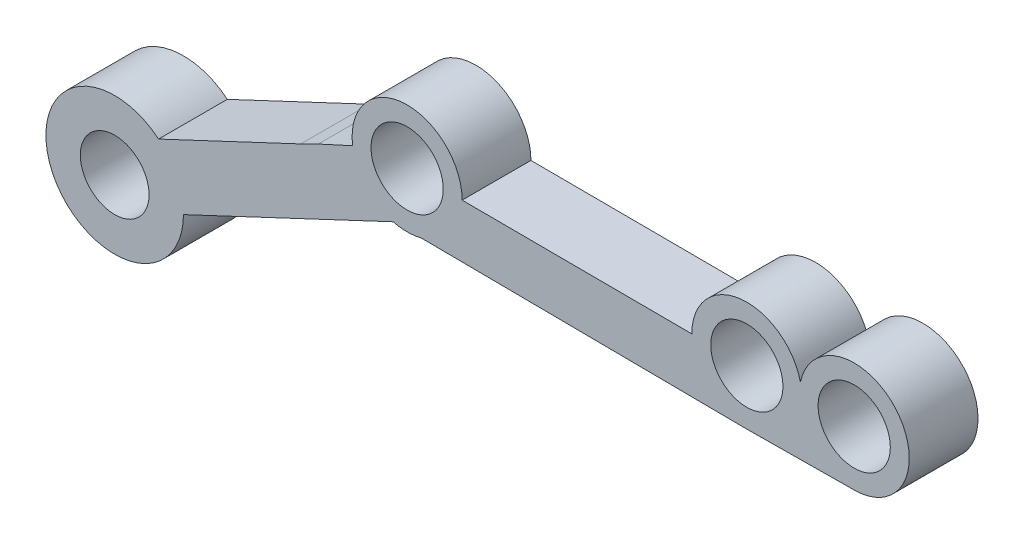
SolidWorks part; units mm, degrees
ref_plane "Front Plane" through (0, 0, 0) normal (0, 0, 1) x (1, 0, 0)
ref_plane "Top Plane" through (0, 0, 0) normal (0, 1, 0) x (1, 0, 0)
ref_plane "Right Plane" through (0, 0, 0) normal (1, 0, 0) x (0, 0, -1)
other "Configuration Table"
sketch "Sketch1" plane through (0, 0, 0) normal (0, 0, 1) x (1, 0, 0)
  line L0 (0, 0) -> (34, 0)
  line L1 (0, 0) -> (0, -15) construction
  line L2 (0, -15) -> (0, 0) construction
  line L3 (-12.0934, -8.0179) -> (-9.4868, -9.5228)
  line L4 (0, -5) -> (34, -5)
  line L5 (35, -4) -> (35, -1)
  arc A0 (0, 0) -> (-12.4215, -6.5913) centre (0, -15) ccw
  arc A1 (0, -5) -> (-8.1698, -9.2334) centre (0, -15) ccw
  arc A2 (34, 0) -> (35, -1) centre (34, -1) cw
  arc A3 (34, -5) -> (35, -4) centre (34, -4) ccw
  arc A4 (-12.4215, -6.5913) -> (-12.0934, -8.0179) centre (-11.5934, -7.1519) ccw
  arc A5 (-8.1698, -9.2334) -> (-9.4868, -9.5228) centre (-8.9868, -8.6567) cw
  dimension "D1" = 1
  dimension "D2" = 1
  dimension "D3" = 1
  dimension "D4" = 1
extrude "Boss-Extrude1" add sketch "Sketch1" along normal blind 5
sketch "Sketch2" plane through (0, 0, 5) normal (0, 0, 1) x (1, 0, 0)
  line L0 (28.5419, -2.571) -> (32.6338, -2.571) construction
  line L1 (-9.5871, -6.6866) -> (-10.7901, -8.7703) construction
  line L2 (-12.0934, -8.0179) -> (-9.4868, -9.5228) construction
  line L3 (32.6338, -2.571) -> (24.6949, -2.571) construction
  circle A0 centre (32.6338, -2.571) radius 1.5
  circle A3 centre (-9.5871, -6.6866) radius 1.5
  circle A4 centre (24.6949, -2.571) radius 1.5
sketch "Sketch3" plane through (0, 0, 0) normal (0, 0, -1) x (-1, 0, 0)
  line L0 (-35, -2.5) -> (0, -2.5) construction
  line L1 (-35, -4) -> (-35, -1) construction
  circle A0 centre (0, -2.5) radius 2.5
extrude "Cut-Extrude3" cut sketch "Sketch3" against normal blind 10
extrude "Cut-Extrude4" cut sketch "Sketch2" against normal blind 7
sketch "Sketch4" plane through (0, 0, 5) normal (0, 0, 1) x (1, 0, 0)
  line L0 (24.6949, -2.571) -> (16.6949, -2.571) construction
  circle A0 centre (16.6949, -2.571) radius 2.5
sketch "Sketch5" plane through (0, 0, 0) normal (0, 0, -1) x (-1, 0, 0)
  circle A0 centre (0, -2.5) radius 4
extrude "Boss-Extrude2" add sketch "Sketch5" against normal blind 5
sketch "Sketch6" plane through (0, 0, 5) normal (0, 0, 1) x (1, 0, 0)
  line L0 (35, -2.5) -> (13.021, -2.5) construction
  line L1 (35, -4) -> (35, -1) construction
  line L2 (16.6906, -2.5) -> (16.6906, -5) construction
  line L3 (3.1225, -5) -> (34, -5) construction
  circle A0 centre (16.6906, -2.5) radius 4
extrude "Boss-Extrude3" add sketch "Sketch6" against normal through all
sketch "Sketch7" plane through (0, 0, 5) normal (0, 0, 1) x (1, 0, 0)
  line L0 (35, -2.5) -> (32.5, -2.5)
  line L1 (35, -4) -> (35, -1) construction
  circle A0 centre (32.5, -2.5) radius 4
  line M5 (34, 0) -> (19.8131, 0)
  line M17 (19.8131, -5) -> (34, -5)
  arc M18 (34, -5) -> (35, -4) centre (34, -4) ccw
  line M19 (35, -4) -> (35, -1)
  arc M20 (35, -1) -> (34, 0) centre (34, -1) ccw
extrude "Boss-Extrude4" add sketch "Sketch7" against normal through all contours A0 M17 M5 M20 M19 M18
sketch "Sketch9" plane through (0, 0, 5) normal (0, 0, 1) x (1, 0, 0)
  circle A0 centre (-9.5871, -6.6866) radius 4
extrude "Boss-Extrude5" add sketch "Sketch9" against normal through all
sketch "Sketch10" plane through (0, 0, 5) normal (0, 0, 1) x (1, 0, 0)
  circle A0 centre (0, -2.5) radius 2.625
  circle A1 centre (-9.5871, -6.6866) radius 2.625
  circle A2 centre (16.6906, -2.5) radius 2.5
  circle A3 centre (32.5, -2.5) radius 2.625
extrude "Cut-Extrude5" cut sketch "Sketch10" against normal through all
sketch "Sketch11" plane through (0, 0, 5) normal (0, 0, 1) x (1, 0, 0)
  circle A0 centre (24.6949, -2.571) radius 4
  circle A1 centre (24.6949, -2.571) radius 2.5
extrude "Boss-Extrude6" add sketch "Sketch11" against normal through all contours A0
sketch "Sketch12" plane through (0, 0, 5) normal (0, 0, 1) x (1, 0, 0)
  circle A0 centre (24.6949, -2.571) radius 2.625
extrude "Cut-Extrude6" cut sketch "Sketch12" against normal through all
sketch "Sketch13" plane through (0, 0, 5) normal (0, 0, 1) x (1, 0, 0)
  circle A0 centre (16.6906, -2.5) radius 4
extrude "Boss-Extrude7" add sketch "Sketch13" against normal through all
sketch "Sketch14" plane through (0, 0, 5) normal (0, 0, 1) x (1, 0, 0)
  line L0 (13.5681, 0) -> (19.8131, 0)
  line L1 (19.8131, 0) -> (19.6082, 3.1014)
  line L2 (19.6082, 3.1014) -> (13.5681, 2.8442)
  line L3 (13.5681, 2.8442) -> (12.582, 1.2873)
  line L4 (12.582, 1.2873) -> (13.5681, 0)
  line L5 (13.5681, -5) -> (19.8131, -5)
  line L6 (3.1225, -5) -> (13.5681, -5) construction
  line L7 (19.8131, -5) -> (20.9346, -7.6449)
  line L8 (20.9346, -7.6449) -> (15.4424, -9.366)
  line L9 (15.4424, -9.366) -> (11.6327, -7.6449)
  line L10 (11.6327, -7.6449) -> (13.5681, -5)
  arc A0 (13.5681, -5) -> (19.8131, -5) centre (16.6906, -2.5) ccw construction
extrude "Cut-Extrude7" cut sketch "Sketch14" against normal through all
sketch "Sketch15" plane through (0, 0, 5) normal (0, 0, 1) x (1, 0, 0)
  line L0 (-8.7058, -2.7849) -> (-7.6075, 0.7948)
  line L1 (-7.6075, 0.7948) -> (-3.3982, -0.39)
  line L2 (24.6949, -2.571) -> (16.6949, -2.571) construction
  line L3 (4, -2.5) -> (20.6949, -2.571)
  line L4 (21.6305, 0) -> (5.4994, 2.1913)
  line L5 (5.4994, 2.1913) -> (3.1225, 0)
  line L6 (27.7592, 0) -> (28.4537, 2.5282)
  line L7 (28.4537, 2.5282) -> (29.3775, 0)
  arc A0 (-3.3982, -0.39) -> (-2.7655, -5.39) centre (0, -2.5) ccw
  arc A1 (-2.7655, -5.39) -> (-5.5871, -6.7064) centre (0, -15) ccw construction
  arc A2 (-8.7058, -2.7849) -> (-5.5871, -6.7064) centre (-9.5871, -6.6866) cw
  arc A3 (-8.7058, -2.7849) -> (-5.5871, -6.7064) centre (-9.5871, -6.6866) ccw construction
  arc A4 (-6.4564, -4.1969) -> (-3.9614, -3.0543) centre (0, -15) cw
  arc A5 (3.1225, 0) -> (4, -2.5) centre (0, -2.5) cw
  arc A6 (21.6305, 0) -> (20.6949, -2.571) centre (24.6949, -2.571) ccw
  arc A7 (27.7592, 0) -> (28.6949, -2.571) centre (24.6949, -2.571) cw
  arc A8 (29.3775, 0) -> (28.5895, -1.6588) centre (32.5, -2.5) ccw
  arc A9 (29.3775, -5) -> (29.3775, 0) centre (32.5, -2.5) ccw construction
  line M2 (21.6305, 0) -> (3.1225, 0)
  arc M4 (-3.3982, -0.39) -> (-8.7058, -2.7849) centre (0, -15) ccw
  line M12 (29.3775, 0) -> (27.7592, 0)
extrude "Cut-Extrude8" cut sketch "Sketch15" against normal through all contours L4 L5 M2 | A6 A5 L3 M2 | L1 L0 M4 | A2 A4 A0 M4 | L7 L6 M12 | A8 A7 M12
sketch "Sketch16" plane through (0, 0, 5) normal (0, 0, 1) x (1, 0, 0)
  line L0 (1.0127, -6.3697) -> (24.6949, -6.571)
  line L1 (24.6949, -6.571) -> (32.5, -6.5)
  line L2 (32.5, -6.5) -> (28.8344, -3.5575)
  line L3 (28.8344, -3.5575) -> (25.8787, -5.379)
  line L4 (25.8787, -5.379) -> (23.3354, -5.379)
  line L5 (23.3354, -5.379) -> (21.3077, -4.2449)
  line L6 (21.3077, -4.2449) -> (3.0238, -3.8668)
  line L7 (3.0238, -3.8668) -> (0.57, -5.379)
  line L8 (0.57, -5.379) -> (-2.8532, -4.6229)
  line L9 (-2.8532, -4.6229) -> (-6.2213, -5.9633)
  line L10 (-6.2213, -5.9633) -> (-6.565, -9.3072)
  arc A0 (-6.565, -9.3072) -> (1.0127, -6.3697) centre (0, -15) cw
  arc A1 (-6.4564, -4.1969) -> (-5.5871, -6.7064) centre (-9.5871, -6.6866) ccw construction
  arc A2 (-2.7655, -5.39) -> (3.1225, -5) centre (0, -2.5) ccw construction
  arc A3 (21.5168, -5) -> (27.8729, -5) centre (24.6949, -2.571) ccw construction
  arc A4 (29.3775, -5) -> (28.5895, -1.6588) centre (32.5, -2.5) ccw construction
extrude "Boss-Extrude8" add sketch "Sketch16" against normal through all
sketch "Sketch17" plane through (0, 0, 0) normal (0, 0, -1) x (-1, 0, 0)
  line L0 (3.9614, -3.0543) -> (13.4954, -7.5382)
  line L1 (1.0127, -6.3697) -> (11.3037, -11.2096)
  line L2 (13.4954, -7.5382) -> (11.3037, -11.2096)
  line L3 (3.9614, -3.0543) -> (1.0127, -6.3697)
  arc A0 (6.565, -9.3072) -> (6.4564, -4.1969) centre (9.5871, -6.6866) ccw construction
  dimension "D1" = 0
extrude "Boss-Extrude9" add sketch "Sketch17" against normal up to surface (5 mm away) up to face at (10.3441, -4.1407, 5)
sketch "Sketch18" plane through (0, 0, 0) normal (0, 0, -1) x (-1, 0, 0)
  line L0 (3.9614, -3.0543) -> (6.4564, -4.1969)
  arc A0 (3.9614, -3.0543) -> (6.4564, -4.1969) centre (0, -15) cw
extrude "Cut-Extrude9" cut sketch "Sketch18" against normal blind 10
sketch "Sketch19" plane through (0, 0, 0) normal (0, 0, -1) x (-1, 0, 0)
  line L0 (6.0017, -8.716) -> (10.1167, -10.6514)
  arc A0 (6.0017, -8.716) -> (10.1167, -10.6514) centre (9.0269, -7.6262) ccw
extrude "Cut-Extrude10" cut sketch "Sketch19" against normal blind 10
sketch "Sketch20" plane through (0, 0, 0) normal (0, 0, -1) x (-1, 0, 0)
  line L0 (6.4564, -4.1969) -> (7.7332, -4.8282)
  line L1 (7.7332, -4.8282) -> (12.2008, -6.9294)
  line L2 (12.2008, -6.9294) -> (14.1057, -7.8252)
  line L3 (14.1057, -7.8252) -> (14.3321, -2.3977)
  line L4 (14.3321, -2.3977) -> (7.6306, -1.4515)
  line L5 (7.6306, -1.4515) -> (6.4564, -4.1969)
extrude "Cut-Extrude11" cut sketch "Sketch20" against normal blind 10
sketch "Sketch21" plane through (0, 0, 0) normal (0, 0, -1) x (-1, 0, 0)
  line L0 (11.3037, -11.2096) -> (13.1146, -7.3591)
  line L4 (1.0127, -6.3697) -> (11.3037, -11.2096) construction
  line L5 (11.3037, -11.2096) -> (12.1913, -9.7228) construction
  line L6 (13.4954, -7.5382) -> (7.7332, -4.8282) construction
  line L7 (13.1146, -7.3591) -> (14.2225, -7.8802)
  line L8 (14.2225, -7.8802) -> (12.354, -11.853)
  line L9 (12.354, -11.853) -> (11.3037, -11.2096)
extrude "Cut-Extrude12" cut sketch "Sketch21" against normal blind 10
sketch "Sketch30" plane through (0, 0, 0) normal (0, 0, -1) x (-1, 0, 0)
  line L0 (13.1146, -7.3591) -> (11.3037, -11.2096)
  line L1 (11.3037, -11.2096) -> (16.2583, -13.5399)
  line L3 (18.0692, -9.6893) -> (13.1146, -7.3591)
  arc A0 (16.2583, -13.5399) -> (18.0692, -9.6893) centre (21.2583, -13.5403) ccw
  circle A1 centre (21.2583, -13.5403) radius 2.5
  dimension "D2" = 10
  dimension "D3" = 5
extrude "Boss-Extrude16" add sketch "Sketch30" against normal up to surface (5 mm away) up to face at (7.566, -4.6083, 5)
